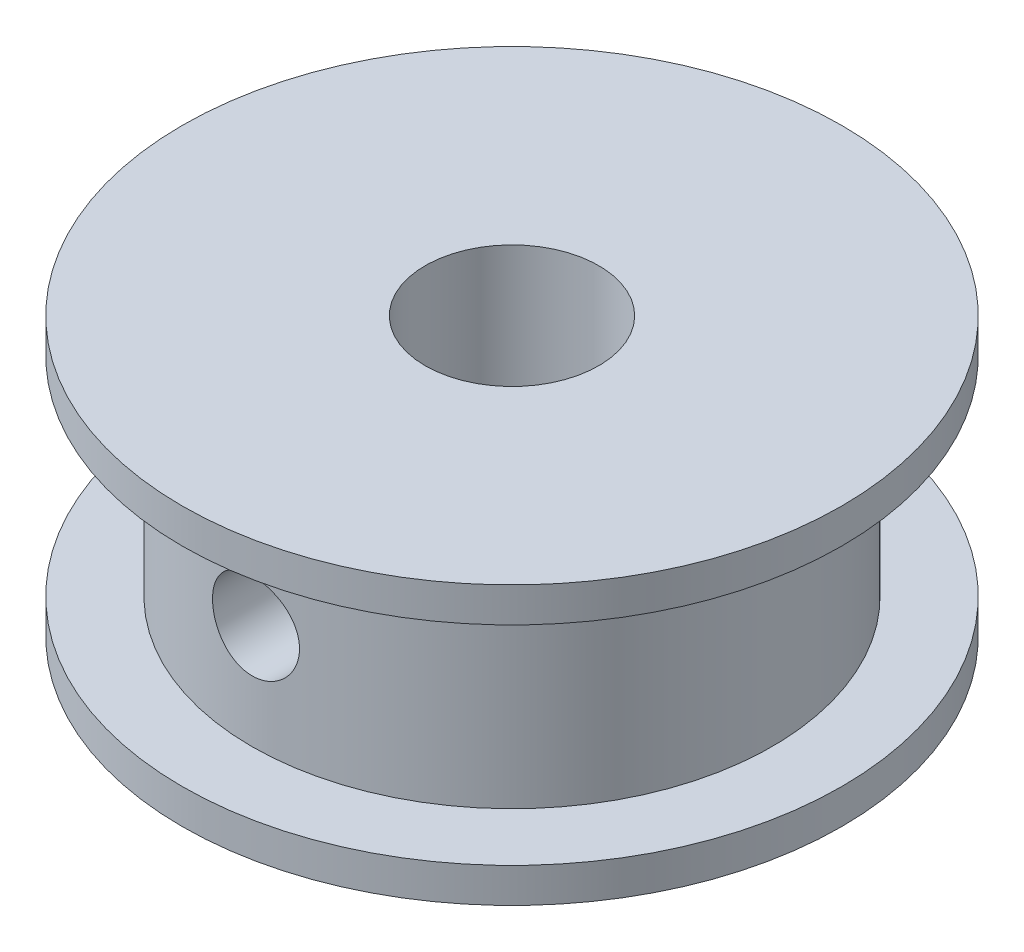
from build123d import *

# Parameters (mm, degrees)
HOLE_WIZARD_M3_1_REACH  = 21.894
HOLE_WIZARD_M3_1_BORE_R = 1.25


with BuildPart() as part:
    # 草图1 → 旋转1 (revolve)
    with BuildSketch(Plane.XY, mode=Mode.PRIVATE) as revolve_1_sk:
        Polygon((9.5, 9.117025796), (2.5, 9.117025796), (2.5, 1.117025796), (9.5, 1.117025796), (9.5, 2.117025796), (7.5, 2.117025796), (7.5, 8.117025796), (9.5, 8.117025796), align=None)
    revolve(revolve_1_sk.sketch.rotate(Axis((0, 18.913531016, 0), (0, -1, 0)), 90), axis=Axis((0, 18.913531016, 0), (0, -1, 0)))

    # M3 螺纹孔1 bore (on position points) → M3 螺纹孔1 (cut, up to next)
    with BuildSketch(Plane(origin=(0.019511296, 5.135461688, 7.499974621), x_dir=(0.999996616077, 0, -0.002601506145), z_dir=(0.002601506145, 0, 0.999996616077)), mode=Mode.PRIVATE) as hole_wizard_m3_1_sk1:
        Circle(HOLE_WIZARD_M3_1_BORE_R)
    hole_wizard_m3_1_tool1 = extrude(hole_wizard_m3_1_sk1.sketch, amount=-HOLE_WIZARD_M3_1_REACH, mode=Mode.PRIVATE) & part.part
    add(hole_wizard_m3_1_tool1.solids().sort_by_distance((0.019511, 5.135462, 7.499975))[0], mode=Mode.SUBTRACT)


solid = part.part
